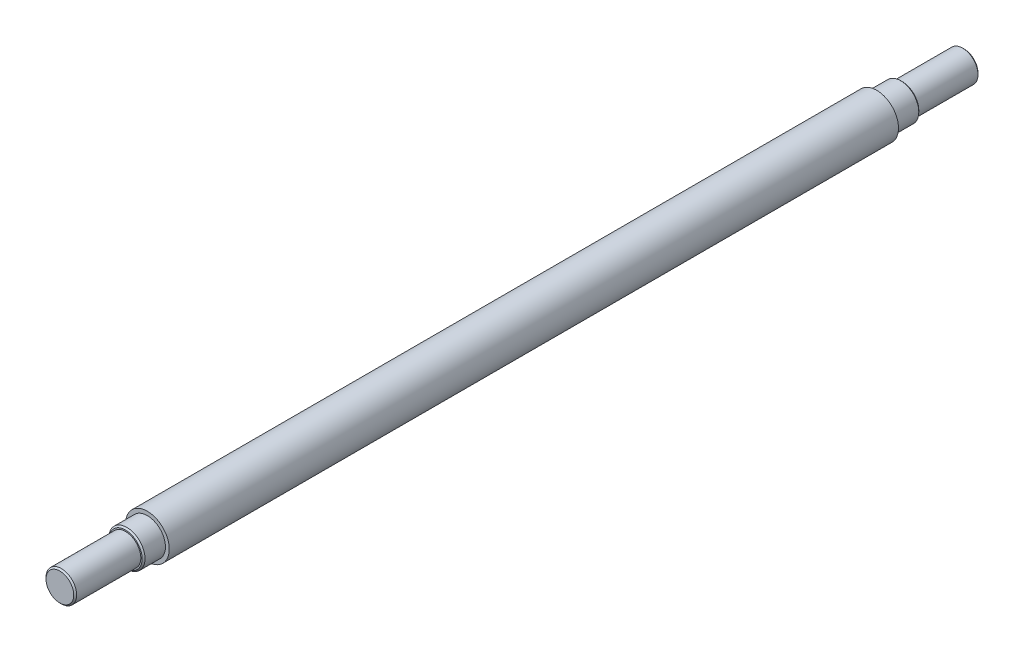
SolidWorks part; units mm, degrees
ref_plane "Front Plane" through (0, 0, 0) normal (0, 0, 1) x (1, 0, 0)
ref_plane "Top Plane" through (0, 0, 0) normal (0, 1, 0) x (1, 0, 0)
ref_plane "Right Plane" through (0, 0, 0) normal (1, 0, 0) x (0, 0, -1)
sketch "Sketch1" plane through (0, 0, 0) normal (0, 0, 1) x (1, 0, 0)
  circle A0 centre (0, 0) radius 21
  dimension "D1" = 42
extrude "Boss-Extrude1" add sketch "Sketch1" along normal blind 85
sketch "Sketch2" plane through (0, 0, 85) normal (0, 0, 1) x (1, 0, 0)
  circle A0 centre (0, 0) radius 24.8
  dimension "D1" = 49.6
extrude "Boss-Extrude2" add sketch "Sketch2" along normal blind 35
sketch "Sketch3" plane through (0, 0, 120) normal (0, 0, 1) x (1, 0, 0)
  circle A0 centre (0, 0) radius 30
  dimension "D1" = 60
extrude "Boss-Extrude3" add sketch "Sketch3" along normal blind 1000
sketch "Sketch4" plane through (0, 0, 1120) normal (0, 0, 1) x (1, 0, 0)
  circle A0 centre (0, 0) radius 24.8
  dimension "D1" = 49.6
extrude "Boss-Extrude4" add sketch "Sketch4" along normal blind 30
sketch "Sketch5" plane through (0, 0, 1150) normal (0, 0, 1) x (1, 0, 0)
  circle A0 centre (0, 0) radius 21
  dimension "D1" = 42
extrude "Boss-Extrude5" add sketch "Sketch5" along normal blind 90
chamfer "Chamfer2" distance 2 angle 45 4 edges at (21, 0, 1240) (24.8, 0, 85) (21, 0, 0) (24.8, 0, 1150)
